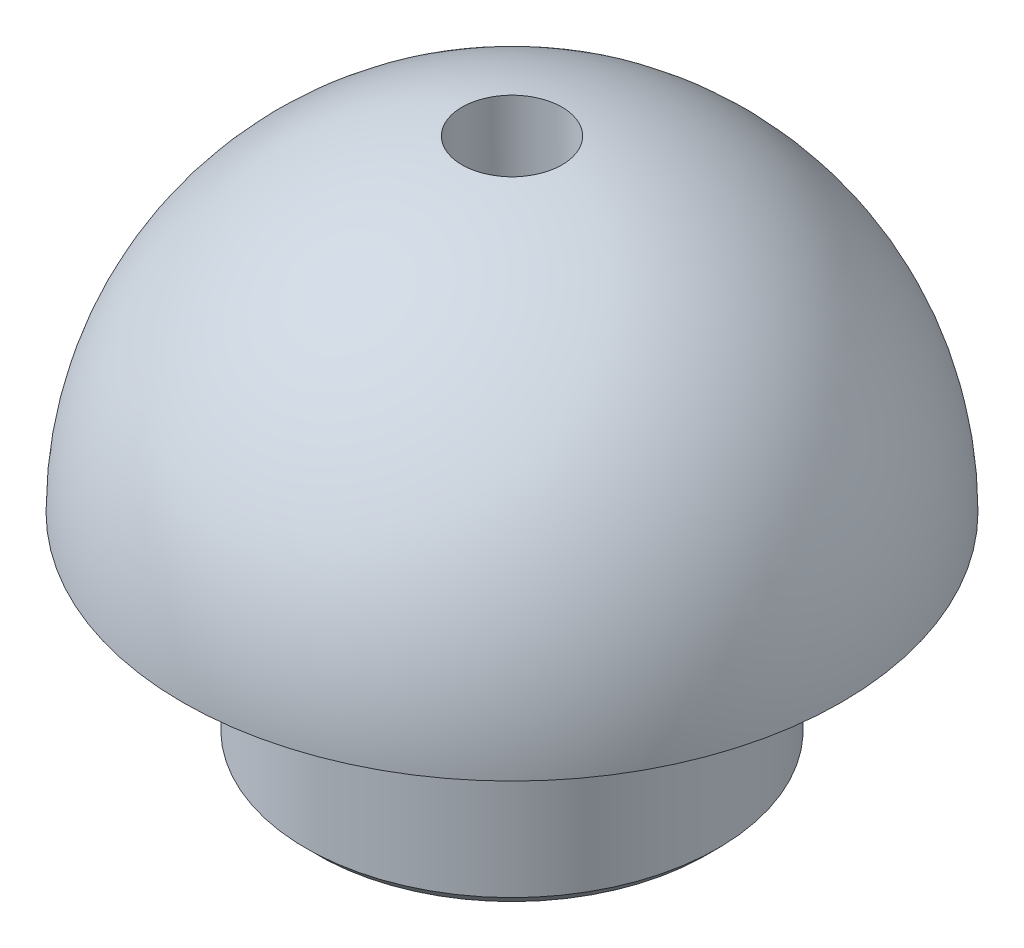
SolidWorks part; units mm, degrees
material "45"
ref_plane "前视基准面" through (0, 0, 0) normal (0, 0, 1) x (1, 0, 0)
ref_plane "上视基准面" through (0, 0, 0) normal (0, 1, 0) x (1, 0, 0)
ref_plane "右视基准面" through (0, 0, 0) normal (1, 0, 0) x (0, 0, -1)
sketch "草图1" plane through (0, 0, 0) normal (0, 0, 1) x (1, 0, 0)
  line L0 (17.5, 0) -> (28, 0)
  line L1 (0, 0) -> (0, 28)
  line L2 (0, 0) -> (0, -17)
  line L3 (0, -17) -> (17.5, -17)
  line L4 (17.5, -17) -> (17.5, 0)
  arc A0 (28, 0) -> (0, 28) centre (0, 0) ccw
  dimension "D1" = 28
  dimension "D2" = 17
  dimension "D3" = 17.5
revolve "旋转1" add sketch "草图1" angle 360 about L1
ref_plane "基准面1" through (0, 28, 0) normal (0, 1, 0) x (1, 0, 0)
hole_wizard "M10 螺纹孔1" positions "草图2" profile "草图3" tap size "M10" standard "GB"
sketch "草图2" plane through (0, 28, 0) normal (0, 1, 0) x (1, 0, 0)
  point P0 (0, 0)
sketch "草图3" plane through (0, 28, 0) normal (1, 0, 0) x (0, 0, 1)
  line L0 (0, 0) -> (0, 14.5537)
  line L1 (0, 14.5537) -> (4.25, 12)
  line L2 (4.25, 12) -> (4.25, 0)
  line L5 (4.25, 0) -> (0, 0)
  line L10 (0, 14.5537) -> (-4.25, 12) construction
  line L11 (0, -6.35) -> (0, 107.95) construction
  dimension "螺纹孔钻头直径" = 8.5
  dimension "螺纹孔钻头深度" = 12
  dimension "导头角度" = 118
cosmetic thread "孔螺蚊线1" parameters "D1"=12, "D2"=10
chamfer "倒角1" distance 1 angle 45 1 edges at (0, -17, -17.5)
